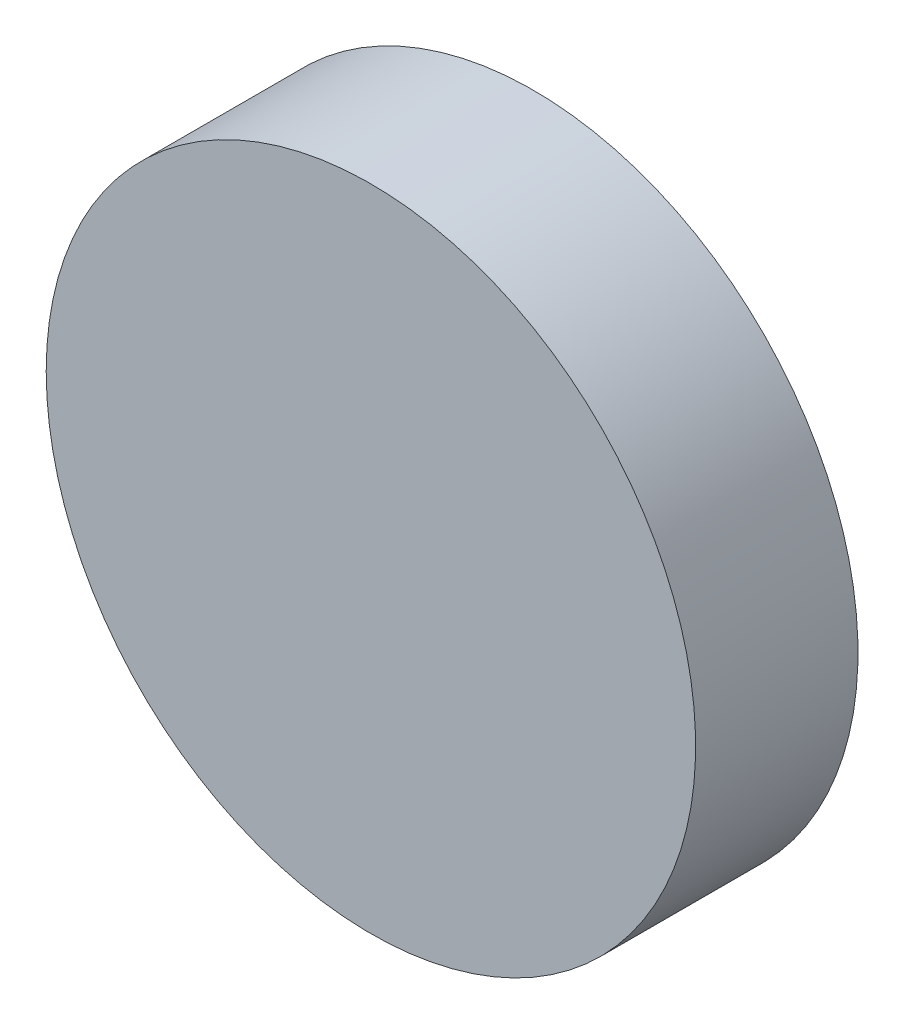
SolidWorks part; units mm, degrees
ref_plane "Front Plane" through (0, 0, 0) normal (0, 0, 1) x (1, 0, 0)
ref_plane "Top Plane" through (0, 0, 0) normal (0, 1, 0) x (1, 0, 0)
ref_plane "Right Plane" through (0, 0, 0) normal (1, 0, 0) x (0, 0, -1)
sketch "Sketch1" plane through (0, 0, 0) normal (0, 0, 1) x (1, 0, 0)
  circle A0 centre (0, 0) radius 19.05
  dimension "D1" = 38.1
extrude "Boss-Extrude1" add sketch "Sketch1" along normal blind 9.525
sketch "Sketch2" plane through (0, 0, 9.525) normal (0, 0, 1) x (1, 0, 0)
  point P0 (0, 0)
sketch "Sketch3" plane through (0, 0, 0) normal (0, 0, -1) x (-1, 0, 0)
  point P0 (0, 0)
